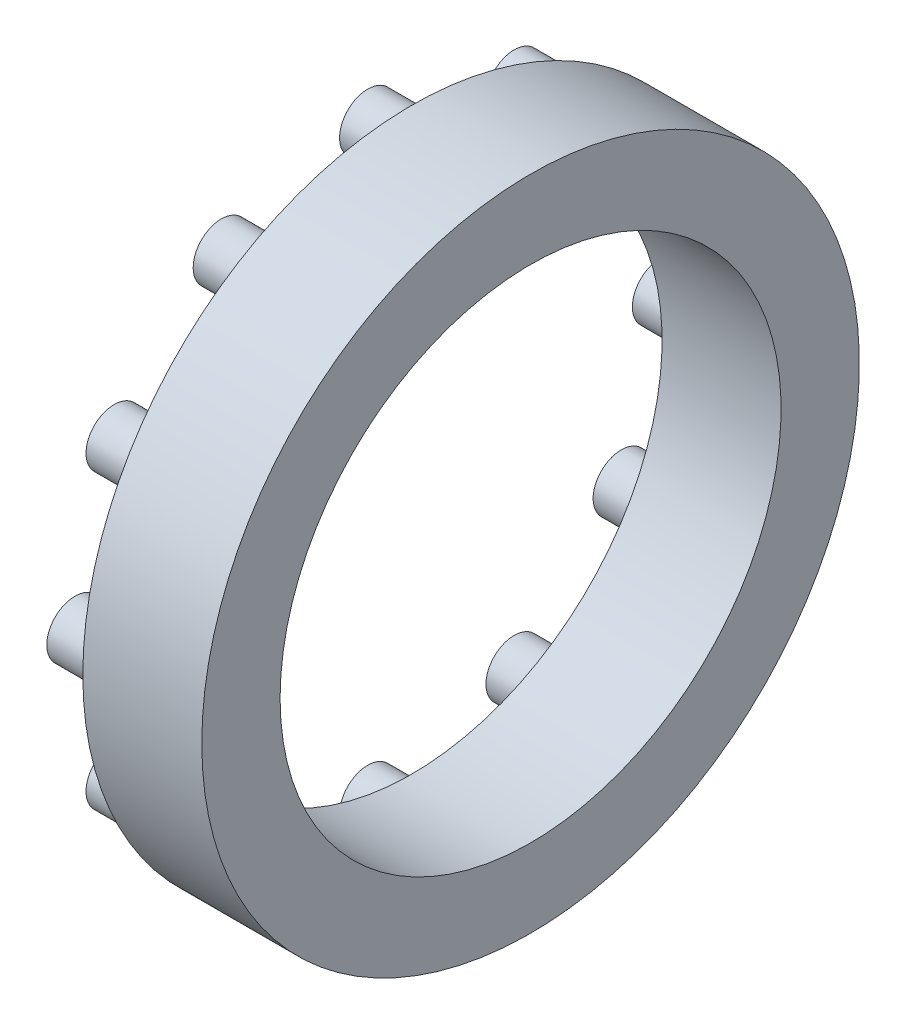
from build123d import *

# Parameters (mm, degrees)
SKETCH1_W           = 38
SKETCH1_H           = 25
SKETCH2_R           = 9
BOSS_EXTRUDE1_DEPTH = 14
CIRPATTERN1_COUNT   = 12


with BuildPart() as part:
    # Sketch1 → Revolve1 (revolve)
    with BuildSketch(Plane.XY, mode=Mode.PRIVATE) as revolve1_sk:
        with Locations((19, 92.5)):
            Rectangle(SKETCH1_W, SKETCH1_H)
    revolve(revolve1_sk.sketch.rotate(Axis((0, 0, 0), (1, 0, 0)), 90), axis=Axis((0, 0, 0), (1, 0, 0)))

    # Sketch2 → Boss-Extrude1 (add)
    with BuildSketch(Plane.ZY):
        with Locations(Location((0, 93.5, 0), (0, 0, 180))):
            Circle(SKETCH2_R)
        Polygon((5.715, 93.5), (2.8575, 98.449335183), (-2.8575, 98.449335183), (-5.715, 93.5), (-2.8575, 88.550664817), (2.8575, 88.550664817), align=None, mode=Mode.SUBTRACT)
    boss_extrude1 = extrude(amount=BOSS_EXTRUDE1_DEPTH)

    # CirPattern1: Boss-Extrude1 ×12 about axis
    cirpattern1_axis = Axis((0, 0, 0), (1, 0, 0))
    for i in range(1, CIRPATTERN1_COUNT):
        add(boss_extrude1.rotate(cirpattern1_axis, i * 360 / CIRPATTERN1_COUNT))


solid = part.part
